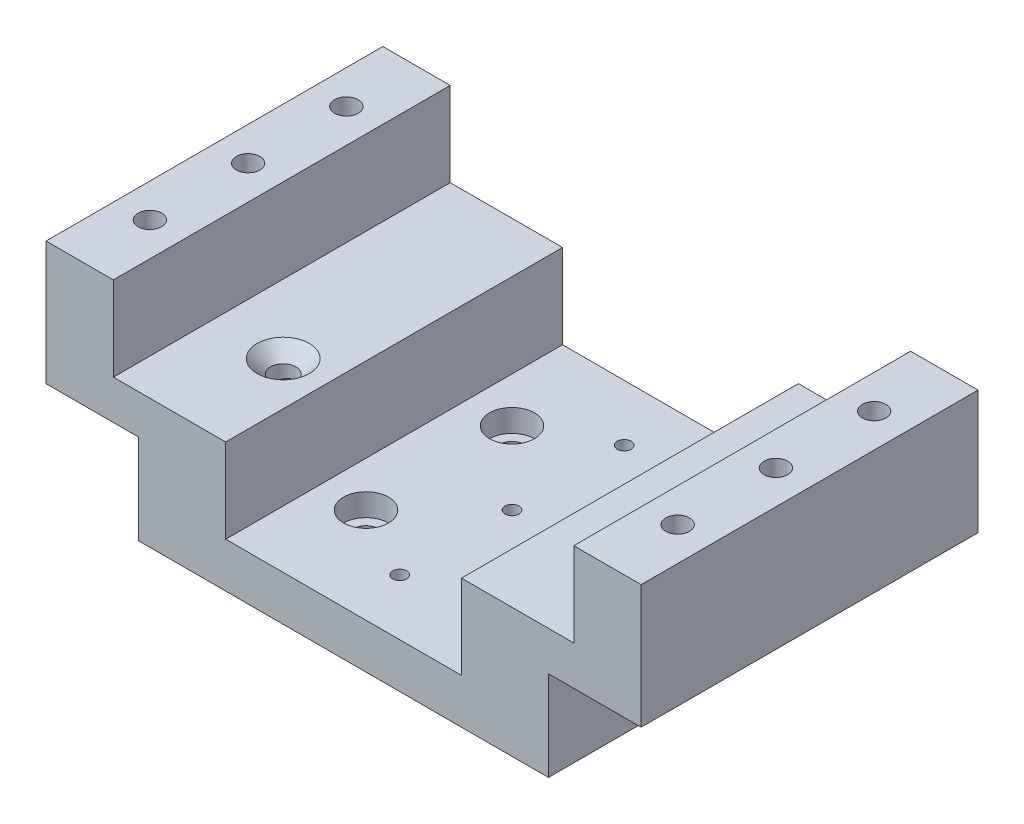
SolidWorks part; units mm, degrees
material "GY-D-73HK"
ref_plane "前视基准面" through (0, 0, 0) normal (0, 0, 1) x (1, 0, 0)
ref_plane "上视基准面" through (0, 0, 0) normal (0, 1, 0) x (1, 0, 0)
ref_plane "右视基准面" through (0, 0, 0) normal (1, 0, 0) x (0, 0, -1)
sketch "草图1" plane through (0, 0, 0) normal (0, 0, 1) x (1, 0, 0)
  line L0 (0, 0) -> (0, 29.641) construction
  line L1 (36.5, 0) -> (-36.5, 0)
  line L2 (-36.5, 0) -> (-36.5, 16)
  line L3 (-36.5, 16) -> (-53, 16)
  line L4 (-53, 16) -> (-53, 38)
  line L5 (-53, 38) -> (-41, 38)
  line L6 (-41, 38) -> (-41, 23)
  line L7 (-41, 23) -> (-21, 23)
  line L8 (-21, 23) -> (-21, 8)
  line L9 (-21, 8) -> (21, 8)
  line L10 (21, 23) -> (21, 8)
  line L11 (41, 23) -> (21, 23)
  line L12 (41, 38) -> (41, 23)
  line L13 (53, 38) -> (41, 38)
  line L14 (53, 16) -> (53, 38)
  line L15 (36.5, 16) -> (53, 16)
  line L16 (36.5, 0) -> (36.5, 16)
  point P13 (0, 8)
  dimension "D1" = 42
  dimension "D2" = 73
  dimension "D3" = 38
  dimension "D4" = 22
  dimension "D5" = 12
  dimension "D6" = 15
  dimension "D7" = 8
  dimension "D8" = 106
extrude "凸台-拉伸1" add sketch "草图1" along normal mid plane 60
hole_wizard "M5 螺纹孔1" positions "草图10" profile "草图9" tap size "M5" standard "GB"
sketch "草图10" plane through (0, 38, 0) normal (0, 1, 0) x (1, 0, 0)
  line L0 (-47, 17.5) -> (-47, -17.5) construction
  line L1 (-47, 0) -> (0, 0) construction
  point P0 (-47, 17.5)
  point P2 (-47, -17.5)
  point P15 (-47, 0)
  dimension "D1" = 47
  dimension "D3" = 35
sketch "草图9" plane through (-47, 38, -17.5) normal (1, 0, 0) x (0, 0, 1)
  line L0 (0, 0) -> (0, 15.6618)
  line L1 (0, 15.6618) -> (2.1, 14.4)
  line L2 (2.1, 14.4) -> (2.1, 0)
  line L5 (2.1, 0) -> (0, 0)
  line L10 (0, 15.6618) -> (-2.1, 14.4) construction
  line L11 (0, -6.35) -> (0, 107.95) construction
  dimension "螺纹孔钻头直径" = 4.2
  dimension "螺纹孔钻头深度" = 14.4
  dimension "导头角度" = 118
cosmetic thread "孔螺蚊线1" parameters "D1"=12, "D2"=5
cosmetic thread "孔螺蚊线2" parameters "D1"=12, "D2"=5
cosmetic thread "孔螺蚊线16" parameters "D1"=12, "D2"=5
mirror "镜向1" about plane through (0, 0, 0) normal (1, 0, 0) of "M5 螺纹孔1"
sketch "草图15" plane through (0, 0, 30) normal (0, 0, 1) x (1, 0, 0)
  line L0 (21, 8) -> (-21, 8) construction
  line L1 (-25, 55.5494) -> (25, 55.5494)
  line L2 (-25, 55.5494) -> (-25, 8)
  line L3 (-25, 8) -> (25, 8)
  line L4 (25, 55.5494) -> (25, 8)
  line L5 (-25, 55.5494) -> (25, 8) construction
  line L6 (-25, 8) -> (25, 55.5494) construction
  line L7 (-21, 8) -> (-21, 23) construction
  point P0 (0, 31.7747)
  dimension "D1" = 4
extrude "切除-拉伸7" cut sketch "草图15" against normal through all
hole_wizard "打孔尺寸(%根据)开槽圆柱头螺钉的类型2" positions "草图21" profile "草图20" counterbore size "M4" standard "GB" end condition through all
sketch "草图21" plane through (0, 8, 0) normal (0, 1, 0) x (1, 0, 0)
  line L0 (-13, 13) -> (13, 13) construction
  line L1 (13, 13) -> (13, -13) construction
  line L4 (0, 0) -> (13, 0) construction
  line L7 (-53, -30) -> (-53, 30) construction
  point P0 (-13, 13)
  point P2 (13, 13)
  point P4 (-13, -13)
  point P6 (13, -13)
  dimension "D1" = 66
  dimension "D2" = 26
  dimension "D3" = 26
sketch "草图20" plane through (-13, 8, -13) normal (1, 0, 0) x (0, 0, 1)
  line L0 (0, 0) -> (0, 8)
  line L1 (0, 8) -> (2.25, 8)
  line L3 (2.25, 8) -> (2.25, 4)
  line L4 (2.25, 4) -> (4, 4)
  line L5 (4, 4) -> (4, 0)
  line L7 (4, 0) -> (0, 0)
  line L11 (0, -6.35) -> (0, 107.95) construction
  dimension "通孔孔直径" = 4.5
  dimension "通孔孔深度" = 8
  dimension "柱形沉头孔直径" = 8
  dimension "柱形沉头孔深度" = 4
hole_wizard "M3 螺纹孔4" positions "草图27" profile "草图26" tap size "M3" standard "GB"
sketch "草图27" plane through (0, 0, -30) normal (0, 0, -1) x (-1, 0, 0)
  line L0 (53, 38) -> (53, 16) construction
  line L1 (-25, 8) -> (25, 8) construction
  point P0 (8, 4)
  point P2 (-7, 4)
  dimension "D1" = 45
  dimension "D2" = 15
  dimension "D3" = 4
sketch "草图26" plane through (-8, 4, -30) normal (1, 0, 0) x (0, 1, 0)
  line L0 (0, 0) -> (0, 13.2511)
  line L1 (0, 13.2511) -> (1.25, 12.5)
  line L2 (1.25, 12.5) -> (1.25, 0)
  line L5 (1.25, 0) -> (0, 0)
  line L10 (0, 13.2511) -> (-1.25, 12.5) construction
  line L11 (0, -6.35) -> (0, 107.95) construction
  dimension "螺纹孔钻头直径" = 2.5
  dimension "螺纹孔钻头深度" = 12.5
  dimension "导头角度" = 118
cosmetic thread "孔螺蚊线14" parameters "D1"=10, "D2"=3
cosmetic thread "孔螺蚊线15" parameters "D1"=10, "D2"=3
sketch "草图29" plane through (0, 0, -30) normal (0, 0, -1) x (-1, 0, 0)
  line L1 (-17.1, -2) -> (17.1, -2)
  line L2 (-17.1, -2) -> (-17.1, 2)
  line L3 (-17.1, 2) -> (17.1, 2)
  line L4 (17.1, -2) -> (17.1, 2)
  line L5 (-17.1, -2) -> (17.1, 2) construction
  line L6 (-17.1, 2) -> (17.1, -2) construction
  point P0 (0, 0)
  dimension "D1" = 34.2
  dimension "D2" = 4
extrude "切除-拉伸9" [suppressed] cut sketch "草图29" against normal blind 238
hole_wizard "M3 螺纹孔5" positions "3D草图2" profile "草图31" tap size "M3" standard "GB" end condition through all
sketch3d "3D草图2"
  line L0 (25, 8, 30) -> (-25, 8, 30) construction
  point P0 (0, 8, 20)
  dimension "D1" = 10
  dimension "D2" = 25
sketch "草图31" plane through (0, 8, 20) normal (1, 0, 0) x (0, 0, 1)
  line L0 (0, 0) -> (0, 8)
  line L1 (0, 8) -> (1.25, 8)
  line L2 (1.25, 8) -> (1.25, 0)
  line L5 (1.25, 0) -> (0, 0)
  line L11 (0, -6.35) -> (0, 107.95) construction
  dimension "通孔螺纹孔钻头直径" = 2.5
  dimension "通孔螺纹孔钻头深度" = 8
cosmetic thread "孔螺蚊线17" parameters "D2"=3
pattern_linear "阵列(线性)1" count 3 spacing 20 along (0, 0, -1) of "M3 螺纹孔5"
hole_wizard "M3 螺纹孔6" positions "3D草图4" profile "草图34" tap size "M3" standard "GB"
sketch3d "3D草图4"
  line L0 (25, 8, -30) -> (25, 23, -30) construction
  point P0 (33, 18, -30)
  point P2 (33, 12, -30)
  dimension "D1" = 8
  dimension "D3" = 5
  dimension "D4" = 6
sketch "草图34" plane through (33, 18, -30) normal (1, 0, 0) x (0, 1, 0)
  line L0 (0, 0) -> (0, 9.2511)
  line L1 (0, 9.2511) -> (1.25, 8.5)
  line L2 (1.25, 8.5) -> (1.25, 0)
  line L5 (1.25, 0) -> (0, 0)
  line L10 (0, 9.2511) -> (-1.25, 8.5) construction
  line L11 (0, -6.35) -> (0, 107.95) construction
  dimension "螺纹孔钻头直径" = 2.5
  dimension "螺纹孔钻头深度" = 8.5
  dimension "导头角度" = 118
cosmetic thread "孔螺蚊线18" parameters "D1"=6, "D2"=3
cosmetic thread "孔螺蚊线19" parameters "D1"=6, "D2"=3
other "移动面1" face at (-25, 15.5, 0) face at (25, 15.5, 0) parameters "D1"=4
sketch "草图37" plane through (0, 0, -30) normal (0, 0, -1) x (-1, 0, 0)
  line L1 (21, 8) -> (21, 23) construction
  line L2 (21, 23) -> (41, 23) construction
  circle A0 centre (28.75, 13) radius 5.5
  dimension "D2" = 11
  dimension "D3" = 10
  dimension "D1" = 7.75
extrude "切除-拉伸10" cut sketch "草图37" against normal blind 50
chamfer "倒角2" distance 1 angle 45 1 edges at (-34.25, 13, -30)
hole_wizard "打孔尺寸(%根据)内六角花形半沉头螺钉的类型1" positions "3D草图5" profile "草图36" countersink size "M6" standard "GB"
sketch3d "3D草图5"
  point P0 (-28.75, 23, 12)
  dimension "D1" = 42
  dimension "D2" = 7.75
sketch "草图36" plane through (-28.75, 23, 12) normal (1, 0, 0) x (0, 0, 1)
  line L0 (0, 0) -> (0, 12.8519)
  line L1 (0, 12.8519) -> (2.25, 11.5)
  line L2 (2.25, 11.5) -> (2.25, 2.4)
  line L3 (2.25, 2.4) -> (4.65, 0)
  line L5 (4.65, 0) -> (0, 0)
  line L6 (-2.25, 2.4) -> (-4.65, 0) construction
  line L10 (0, 12.8519) -> (-2.25, 11.5) construction
  line L11 (0, -6.35) -> (0, 107.95) construction
  dimension "孔直径" = 4.5
  dimension "孔深度" = 11.5
  dimension "近端锥形沉头孔直径" = 9.3
  dimension "近端锥形沉头孔角度" = 90
  dimension "导头角度" = 118
sketch "草图38" plane through (0, 23, 0) normal (0, 1, 0) x (1, 0, 0)
  circle A0 centre (-28.75, -12) radius 0.7077
extrude "切除-拉伸11" cut sketch "草图38" against normal blind 33
hole_wizard "M4 螺纹孔1" positions "3D草图6" profile "草图40" tap size "M4" standard "GB"
sketch3d "3D草图6"
  line L0 (-28.75, 0, 12) -> (-28.75, 7.5, 12) construction
  point P0 (-28.75, 0, 12)
sketch "草图40" plane through (-28.75, 0, 12) normal (1, 0, 0) x (0, 0, -1)
  line L0 (0, 0) -> (0, 11.0914)
  line L1 (0, 11.0914) -> (1.65, 10.1)
  line L2 (1.65, 10.1) -> (1.65, 0.375)
  line L3 (1.65, 0.375) -> (2.025, 0)
  line L5 (2.025, 0) -> (0, 0)
  line L6 (-1.65, 0.375) -> (-2.025, 0) construction
  line L10 (0, 11.0914) -> (-1.65, 10.1) construction
  line L11 (0, -6.35) -> (0, 107.95) construction
  dimension "螺纹孔钻头直径" = 3.3
  dimension "螺纹孔钻头深度" = 10.1
  dimension "近端锥形沉头孔直径" = 4.05
  dimension "近端锥形沉头孔角度" = 90
  dimension "导头角度" = 118
cosmetic thread "孔螺蚊线20" parameters "D1"=7.7533, "D2"=4
